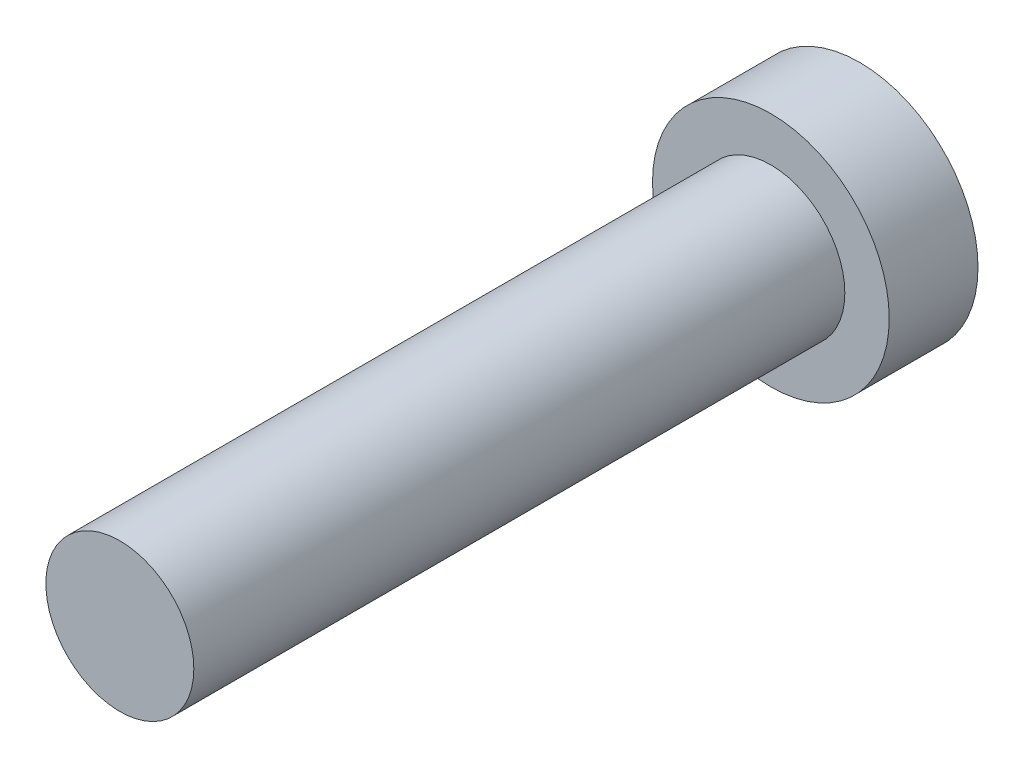
from build123d import *

# Parameters (mm, degrees)
SKETCH1_R           = 25
BOSS_EXTRUDE1_DEPTH = 220
SKETCH2_R           = 40
BOSS_EXTRUDE2_DEPTH = 30


with BuildPart() as part:
    # Sketch1 → Boss-Extrude1 (new body)
    with BuildSketch(Plane.XY):
        Circle(SKETCH1_R)
    extrude(amount=-BOSS_EXTRUDE1_DEPTH)

    # Sketch2 → Boss-Extrude2 (add)
    with BuildSketch(Plane(origin=(0, 0, -220), x_dir=(-1, 0, 0), z_dir=(0, 0, -1))):
        Circle(SKETCH2_R)
    extrude(amount=BOSS_EXTRUDE2_DEPTH)


solid = part.part
